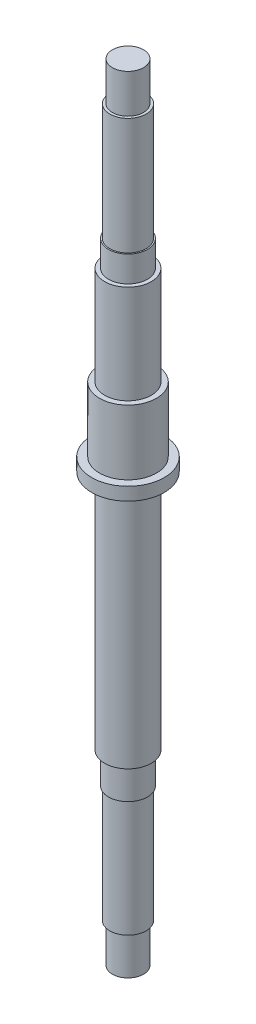
SolidWorks part; units mm, degrees
ref_plane "Front Plane" through (0, 0, 0) normal (0, 0, 1) x (1, 0, 0)
ref_plane "Top Plane" through (0, 0, 0) normal (0, 1, 0) x (1, 0, 0)
ref_plane "Right Plane" through (0, 0, 0) normal (1, 0, 0) x (0, 0, -1)
other "Configuration Table"
sketch "Sketch1" plane through (0, 0, 0) normal (0, 0, 1) x (1, 0, 0)
  line L0 (0, 303) -> (-6, 303)
  line L1 (-6, 288) -> (-6, 303)
  line L2 (-6, 288) -> (-7, 288)
  line L3 (-7, 288) -> (-7, 243)
  line L4 (-7, 243) -> (-7.5, 243)
  line L5 (-7.5, 243) -> (-7.5, 233)
  line L6 (-7.5, 233) -> (-9, 233)
  line L7 (0, 303) -> (0, 0)
  line L8 (-9, 195) -> (-11, 195)
  line L9 (-11, 195) -> (-11, 170)
  line L10 (-11, 170) -> (-14, 170)
  line L13 (-14, 170) -> (-14, 165)
  line L14 (-9, 72) -> (-7.5, 72)
  line L15 (-7.5, 72) -> (-7.5, 60)
  line L16 (-7.5, 60) -> (-7, 60)
  line L17 (-7, 60) -> (-7, 15)
  line L18 (-7, 15) -> (-6, 15)
  line L19 (-6, 15) -> (-6, 0)
  line L20 (-6, 0) -> (0, 0)
  line L21 (0, 303) -> (0, 0) construction
  line L22 (-9, 72) -> (-9, 165)
  line L25 (-14, 165) -> (-9, 165)
  line L28 (-9, 233) -> (-9, 195)
  point P33 (-7.25, 60)
  dimension "D1" = 6
  dimension "D2" = 7
  dimension "D3" = 7.5
  dimension "D4" = 15
  dimension "D5" = 9
  dimension "D6" = 303
  dimension "D7" = 15
  dimension "D8" = 60
  dimension "D9" = 60
  dimension "D10" = 10
  dimension "D11" = 12
  dimension "D12" = 11
  dimension "D13" = 3
  dimension "D14" = 5
  dimension "D15" = 25
  dimension "D16" = 170
revolve "Revolve1" add sketch "Sketch1" angle 360 about L21
